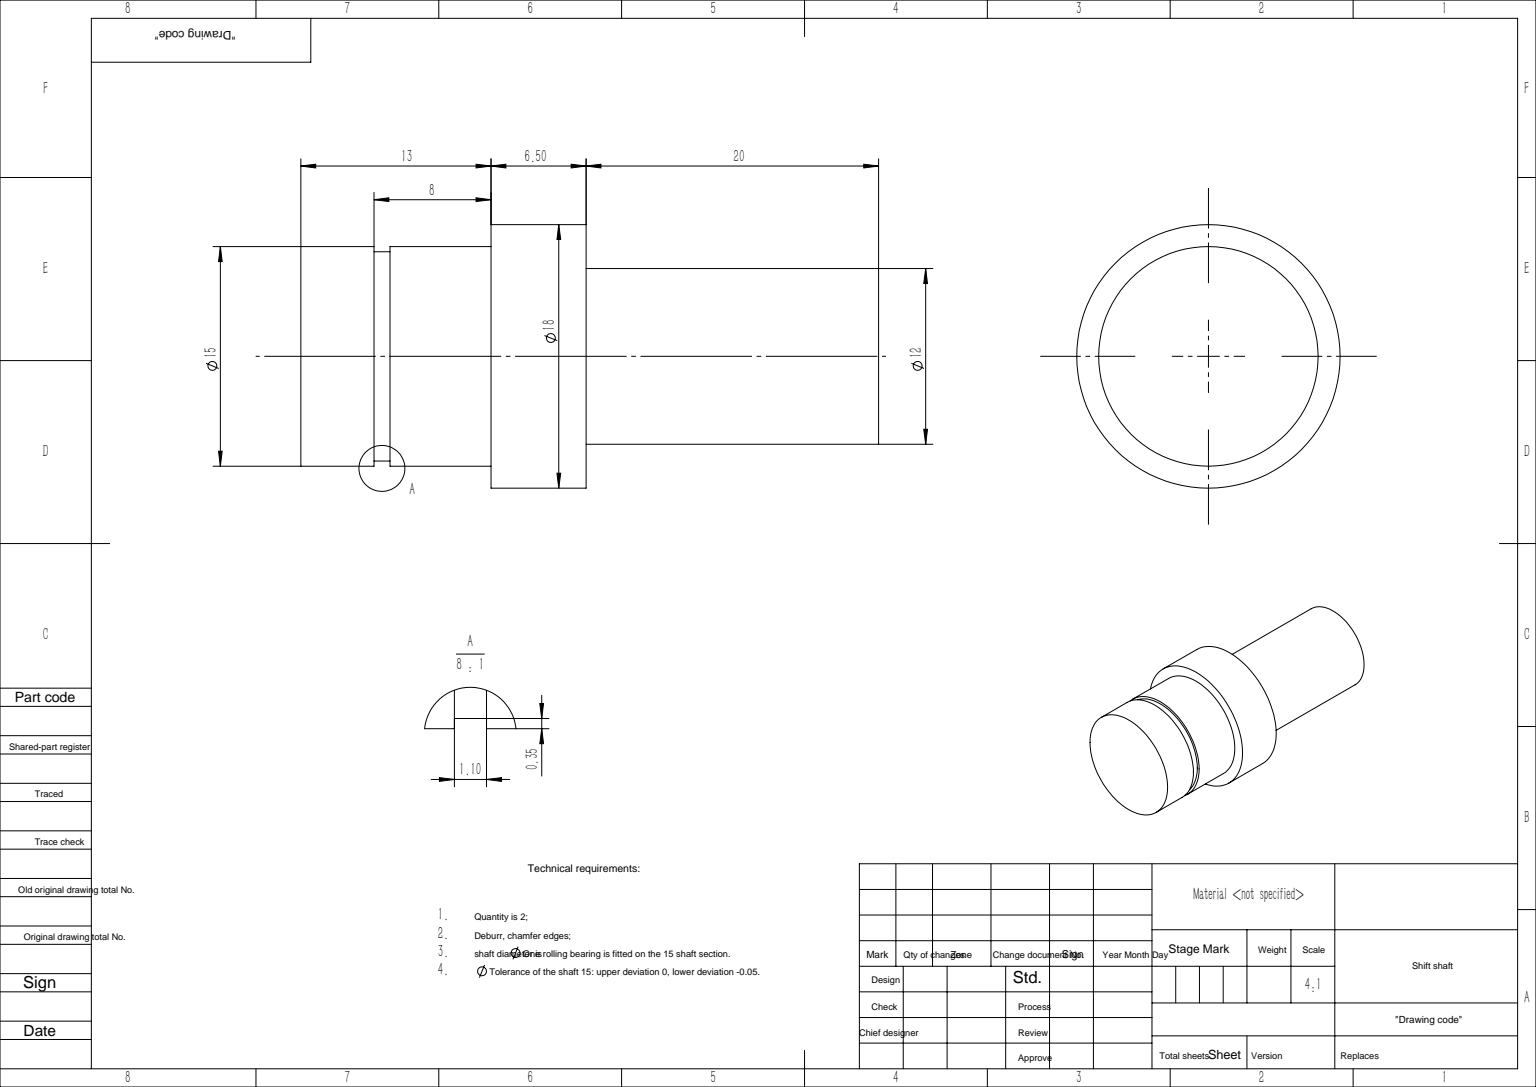
from build123d import *

# Parameters (mm, degrees)
CUT_EXTRUDE_START   = -1.1
SKETCH_3_R          = 7.5
SKETCH_3_R_2        = 7.15
CUT_EXTRUDE_1_DEPTH = 1.1


with BuildPart() as part:
    # 草图2 → 旋转1 (revolve)
    with BuildSketch(Plane(origin=(0, 0, 0), x_dir=(0, 0, -1), z_dir=(1, 0, 0)), mode=Mode.PRIVATE) as revolve_1_sk:
        Polygon((0, 0), (0, 7.5), (13, 7.5), (13, 9), (19.5, 9), (19.5, 6), (39.5, 6), (39.5, 0), align=None)
    revolve(revolve_1_sk.sketch.rotate(Axis((0, 0, -39.5), (0, 0, 1)), 90), axis=Axis((0, 0, -39.5), (0, 0, 1)))

    # 草图3 → 切除-拉伸1 (cut)
    with BuildSketch(Plane.XY.offset(-5).offset(CUT_EXTRUDE_START)):
        with Locations(Location((0, 0, 0), (0, 0, 180))):
            Circle(SKETCH_3_R)
        Circle(SKETCH_3_R_2, mode=Mode.SUBTRACT)
    extrude(amount=CUT_EXTRUDE_1_DEPTH, mode=Mode.SUBTRACT)


solid = part.part
